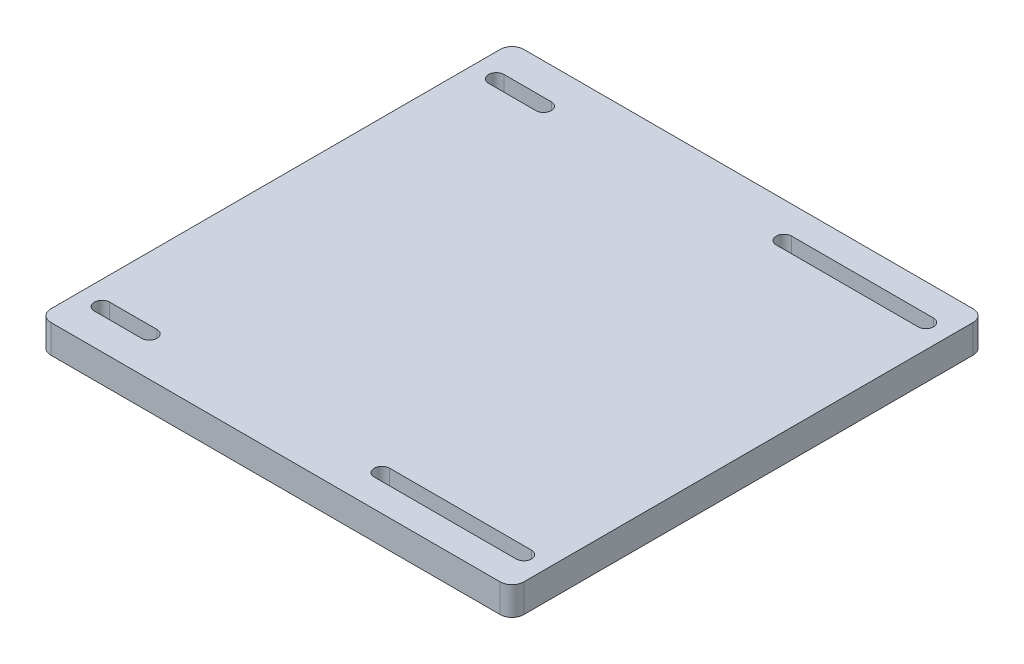
SolidWorks part; units mm, degrees
material "电木（PF）"
ref_plane "前视基准面" through (0, 0, 0) normal (0, 0, 1) x (1, 0, 0)
ref_plane "上视基准面" through (0, 0, 0) normal (0, 1, 0) x (1, 0, 0)
ref_plane "右视基准面" through (0, 0, 0) normal (1, 0, 0) x (0, 0, -1)
sketch "草图1" plane through (0, 0, 0) normal (0, 1, 0) x (1, 0, 0)
  line L1 (-100, 100) -> (100, 100)
  line L2 (-100, 100) -> (-100, -100)
  line L3 (-100, -100) -> (100, -100)
  line L4 (100, 100) -> (100, -100)
  line L5 (-100, 100) -> (100, -100) construction
  line L6 (-100, -100) -> (100, 100) construction
  point P0 (0, 0)
  dimension "D1" = 200
  dimension "D2" = 200
extrude "凸台-拉伸1" add sketch "草图1" along normal blind 12
fillet "圆角1" radius 5 4 edges at (-100, 6, 100) (100, 6, 100) (100, 6, -100) (-100, 6, -100)
sketch "草图2" plane through (0, 12, 0) normal (0, 1, 0) x (1, 0, 0)
  line L0 (-90, 83.375) -> (-70, 83.375) construction
  line L1 (-90, 86.625) -> (-70, 86.625)
  line L2 (-90, 80.125) -> (-70, 80.125)
  line L3 (-100, 95) -> (-100, -95) construction
  line L4 (0, 0) -> (-133.7784, 0) construction
  line L5 (-90, -83.375) -> (-70, -83.375) construction
  line L6 (-90, -86.625) -> (-70, -86.625)
  line L7 (-90, -80.125) -> (-70, -80.125)
  line L8 (0, 0) -> (0, 164.5716) construction
  line L9 (30, 85) -> (90, 85) construction
  line L10 (30, 88.25) -> (90, 88.25)
  line L11 (30, 81.75) -> (90, 81.75)
  line L12 (30, -85) -> (90, -85) construction
  line L13 (30, -88.25) -> (90, -88.25)
  line L14 (30, -81.75) -> (90, -81.75)
  line L15 (100, -95) -> (100, 95) construction
  arc A0 (-90, 86.625) -> (-90, 80.125) centre (-90, 83.375) ccw
  arc A1 (-70, 80.125) -> (-70, 86.625) centre (-70, 83.375) ccw
  arc A2 (-90, -86.625) -> (-90, -80.125) centre (-90, -83.375) cw
  arc A3 (-70, -80.125) -> (-70, -86.625) centre (-70, -83.375) cw
  arc A4 (30, 88.25) -> (30, 81.75) centre (30, 85) ccw
  arc A5 (90, 81.75) -> (90, 88.25) centre (90, 85) ccw
  arc A6 (30, -88.25) -> (30, -81.75) centre (30, -85) cw
  arc A7 (90, -81.75) -> (90, -88.25) centre (90, -85) cw
  point P2 (-80, 83.375)
  point P14 (-80, -83.375)
  point P22 (60, 85)
  point P29 (60, -85)
  dimension "D2" = 3.25
  dimension "D8" = 3.25
  dimension "D1" = 20
  dimension "D3" = 20
  dimension "D4" = 170
  dimension "D5" = 170
  dimension "D6" = 40
  dimension "D7" = 60
extrude "切除-拉伸1" cut sketch "草图2" against normal blind 10
